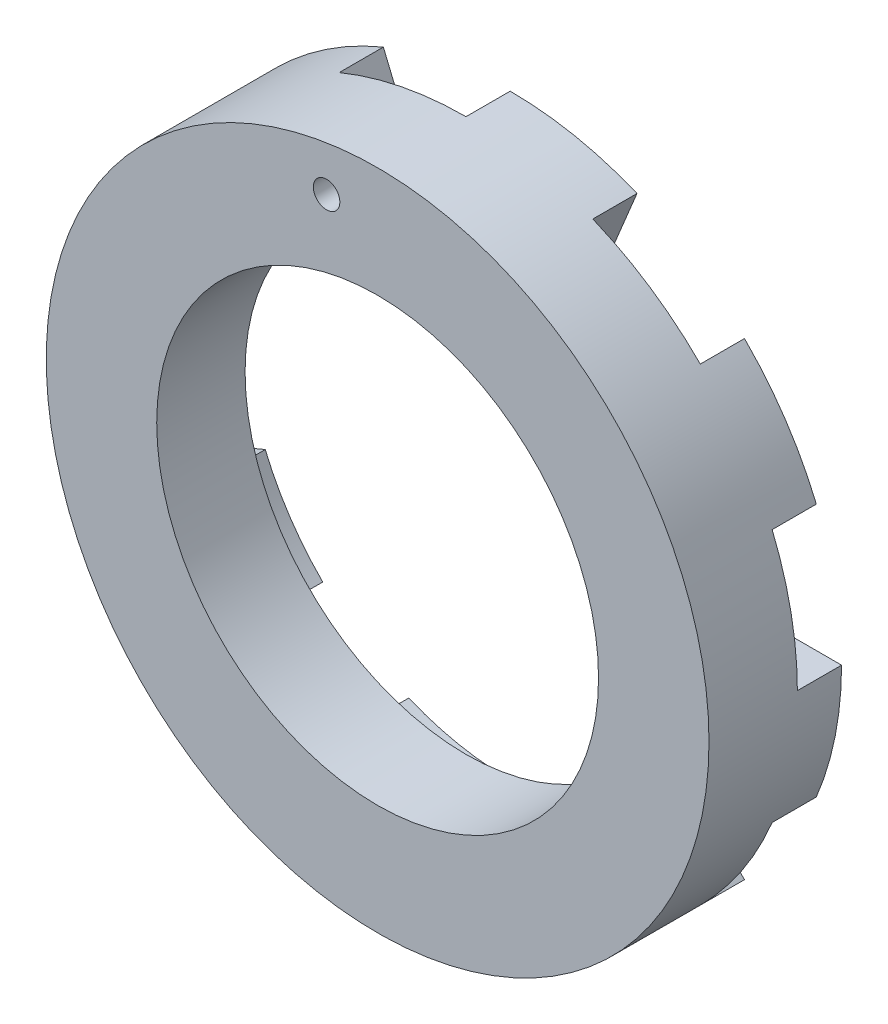
SolidWorks part; units mm, degrees
ref_plane "Front Plane" through (0, 0, 0) normal (0, 0, 1) x (1, 0, 0)
ref_plane "Top Plane" through (0, 0, 0) normal (0, 1, 0) x (1, 0, 0)
ref_plane "Right Plane" through (0, 0, 0) normal (1, 0, 0) x (0, 0, -1)
sketch "Sketch1" plane through (0, 0, 0) normal (0, 0, 1) x (1, 0, 0)
  circle A0 centre (0, 0) radius 25
  circle A1 centre (0, 0) radius 37.5
  dimension "D1" = 50
  dimension "D2" = 75
extrude "Boss-Extrude1" add sketch "Sketch1" along normal blind 15
sketch "Sketch2" plane through (0, 0, 0) normal (0, 0, -1) x (-1, 0, 0)
  circle A0 centre (0, 0) radius 30
  dimension "D1" = 60
extrude "Cut-Extrude1" cut sketch "Sketch2" against normal blind 5
sketch "Sketch3" plane through (0, 0, 0) normal (0, 0, -1) x (-1, 0, 0)
  line L0 (0, 30) -> (0, 37.5)
  line L1 (11.4805, 27.7164) -> (14.3506, 34.6455)
  line L2 (21.2132, 21.2132) -> (26.5165, 26.5165)
  line L3 (27.7164, 11.4805) -> (34.6455, 14.3506)
  line L4 (30, 0) -> (37.5, 0)
  line L5 (27.7164, -11.4805) -> (34.6455, -14.3506)
  line L6 (21.2132, -21.2132) -> (26.5165, -26.5165)
  line L7 (11.4805, -27.7164) -> (14.3506, -34.6455)
  line L8 (0, -30) -> (0, -37.5)
  line L9 (-11.4805, -27.7164) -> (-14.3506, -34.6455)
  line L10 (-21.2132, -21.2132) -> (-26.5165, -26.5165)
  line L11 (-27.7164, -11.4805) -> (-34.6455, -14.3506)
  line L12 (-30, 0) -> (-37.5, 0)
  line L13 (-27.7164, 11.4805) -> (-34.6455, 14.3506)
  line L14 (-21.2132, 21.2132) -> (-26.5165, 26.5165)
  line L15 (-11.4805, 27.7164) -> (-14.3506, 34.6455)
  arc A0 (-14.3506, 34.6455) -> (-26.5165, 26.5165) centre (0, 0) ccw
  arc A1 (-11.4805, 27.7164) -> (-21.2132, 21.2132) centre (0, 0) ccw
  arc A2 (14.3506, 34.6455) -> (0, 37.5) centre (0, 0) ccw
  arc A3 (11.4805, 27.7164) -> (0, 30) centre (0, 0) ccw
  arc A4 (34.6455, 14.3506) -> (26.5165, 26.5165) centre (0, 0) ccw
  arc A5 (27.7164, 11.4805) -> (21.2132, 21.2132) centre (0, 0) ccw
  arc A6 (27.7164, -11.4805) -> (30, 0) centre (0, 0) ccw
  arc A7 (34.6455, -14.3506) -> (37.5, 0) centre (0, 0) ccw
  arc A8 (14.3506, -34.6455) -> (26.5165, -26.5165) centre (0, 0) ccw
  arc A9 (11.4805, -27.7164) -> (21.2132, -21.2132) centre (0, 0) ccw
  arc A10 (-11.4805, -27.7164) -> (0, -30) centre (0, 0) ccw
  arc A11 (-14.3506, -34.6455) -> (0, -37.5) centre (0, 0) ccw
  arc A12 (-34.6455, -14.3506) -> (-26.5165, -26.5165) centre (0, 0) ccw
  arc A13 (-27.7164, -11.4805) -> (-21.2132, -21.2132) centre (0, 0) ccw
  arc A14 (-27.7164, 11.4805) -> (-30, 0) centre (0, 0) ccw
  arc A15 (-34.6455, 14.3506) -> (-37.5, 0) centre (0, 0) ccw
  point P23 (0, 0)
  dimension "D1" = 16
extrude "Cut-Extrude2" cut sketch "Sketch3" against normal blind 5
sketch "Sketch4" plane through (0, 0, 5) normal (0, 0, -1) x (-1, 0, 0)
  circle A0 centre (0, 0) radius 32.5 construction
  circle A1 centre (5.7757, 31.9827) radius 1.5
  dimension "D1" = 65
  dimension "D2" = 3
extrude "Cut-Extrude3" cut sketch "Sketch4" against normal blind 10
